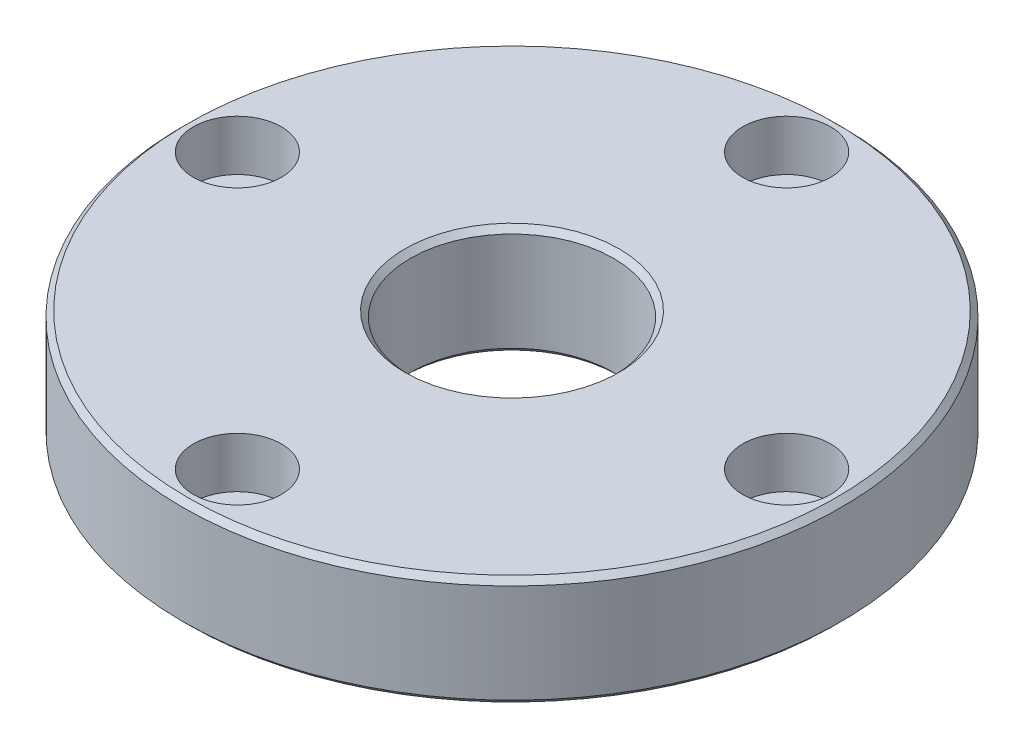
from build123d import *

# Parameters (mm, degrees)
SKETCH_1_R                = 30
EXTRUDE_1_DEPTH           = 10
M20X1_5_1_D               = 18.5
HOLE_WIZARD_1_D           = 4.5
HOLE_WIZARD_1_CBORE_D     = 8
HOLE_WIZARD_1_CBORE_DEPTH = 4.6
CHAMFER_1_SIZE            = 0.5


with BuildPart() as part:
    # 草图1 → 凸台-拉伸1 (new body)
    with BuildSketch(Plane(origin=(0, 0, 0), x_dir=(1, 0, 0), z_dir=(0, 1, 0))):
        with Locations(Location((0, 0, 0), (0, 0, 270))):
            Circle(SKETCH_1_R)
    extrude(amount=EXTRUDE_1_DEPTH)

    # M20x1.5 螺纹孔1 (through all)
    with Locations(Plane(origin=(0, 10, 0), x_dir=(1, 0, 0), z_dir=(0, 1, 0))):
        with Locations((0, 0)):
            Hole(M20X1_5_1_D / 2)

    # 打孔尺寸(%根据)内六角圆柱头螺钉的类型1 (through all)
    with Locations(Plane(origin=(0, 10, 0), x_dir=(1, 0, 0), z_dir=(0, 1, 0))):
        with Locations((0, 25), (25, 0), (0, -25), (-25, 0)):
            CounterBoreHole(HOLE_WIZARD_1_D / 2, HOLE_WIZARD_1_CBORE_D / 2, HOLE_WIZARD_1_CBORE_DEPTH)

    # 倒角1
    chamfer_1_edges = [part.edges().sort_by_distance(p)[0] for p in [
        (0, 0, -30),
        (0, 10, -30),
        (9.25, 10, 0),
        (9.25, 0, 0),
    ]]
    chamfer(chamfer_1_edges, length=CHAMFER_1_SIZE)


solid = part.part
